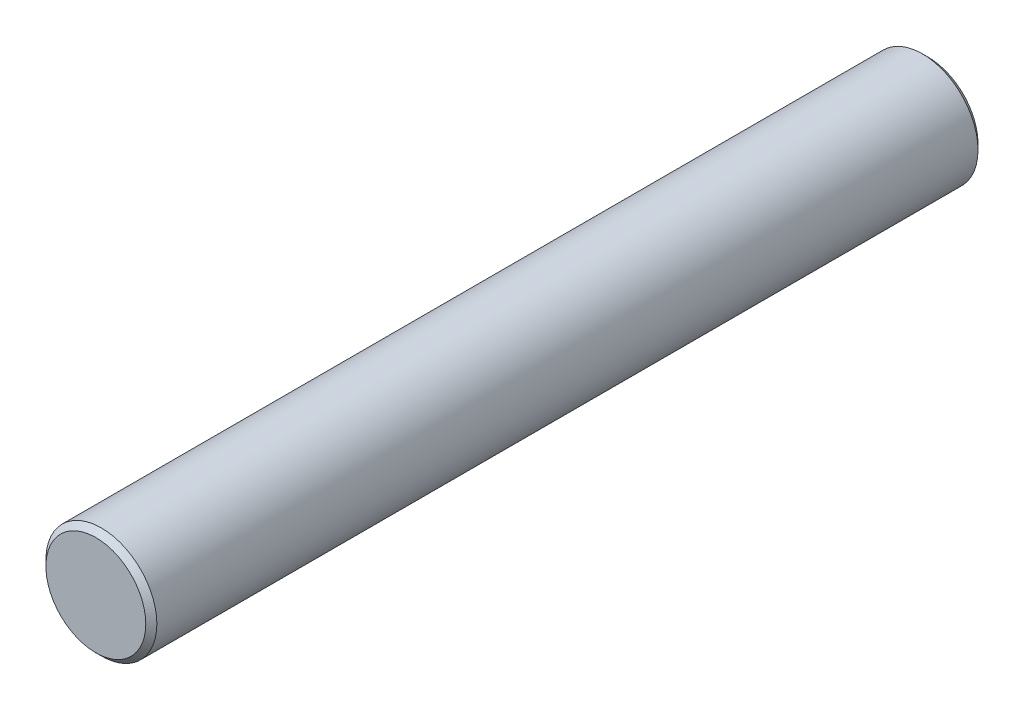
SolidWorks part; units mm, degrees
ref_plane "Front Plane" through (0, 0, 0) normal (0, 0, 1) x (1, 0, 0)
ref_plane "Top Plane" through (0, 0, 0) normal (0, 1, 0) x (1, 0, 0)
ref_plane "Right Plane" through (0, 0, 0) normal (1, 0, 0) x (0, 0, -1)
sketch "Sketch1" plane through (0, 0, 0) normal (0, 0, 1) x (1, 0, 0)
  circle A0 centre (0, 0) radius 10
  dimension "D1" = 20
extrude "Boss-Extrude1" add sketch "Sketch1" against normal blind 150
cosmetic thread "Cosmetic Thread1" parameters "D1"=50, "D2"=17.294
cosmetic thread "Cosmetic Thread2" parameters "D1"=40, "D2"=17.294
chamfer "Chamfer1" distance 1 angle 45 2 edges at (10, 0, -150) (10, 0, 0)
